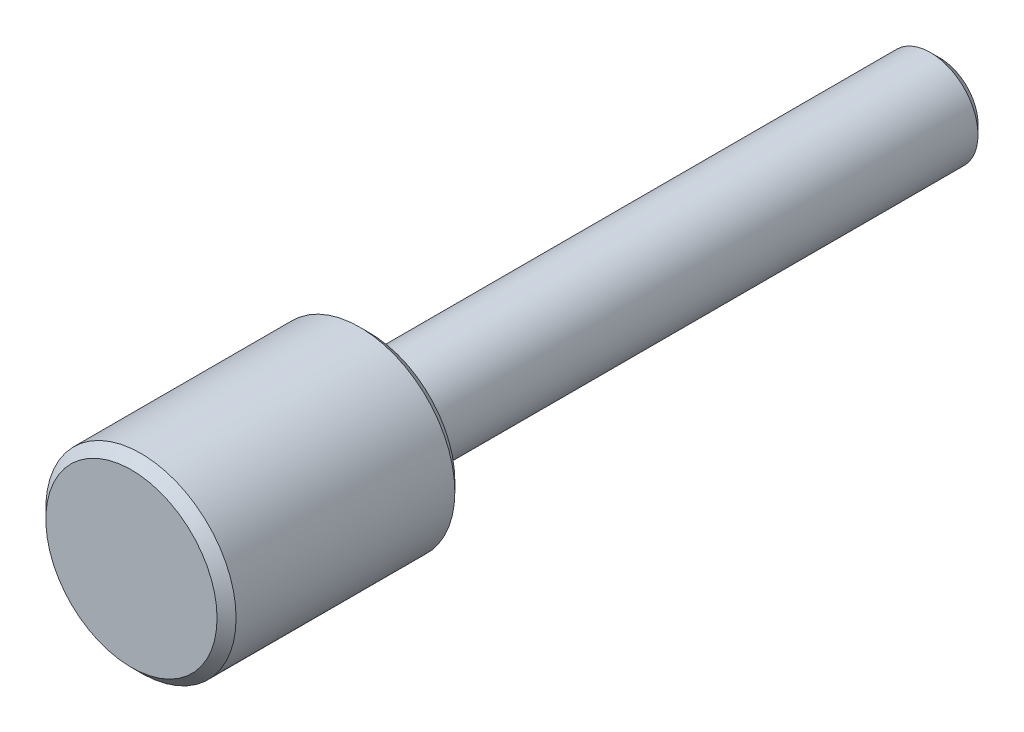
from build123d import *

# Parameters (mm, degrees)
SKETCH1_R           = 1
BOSS_EXTRUDE1_DEPTH = 8.5
SKETCH2_R           = 2
BOSS_EXTRUDE2_DEPTH = 5
CHAMFER1_SIZE       = 0.2


with BuildPart() as part:
    # Sketch1 → Boss-Extrude1 (new, symmetric)
    with BuildSketch(Plane.XY):
        Circle(SKETCH1_R)
    extrude(amount=BOSS_EXTRUDE1_DEPTH, both=True)

    # Sketch2 → Boss-Extrude2 (add)
    with BuildSketch(Plane.XY.offset(8.5)):
        Circle(SKETCH2_R)
    extrude(amount=-BOSS_EXTRUDE2_DEPTH)

    # Chamfer1
    chamfer1_edges = [part.edges().sort_by_distance(p)[0] for p in [
        (-1, 0, -8.5),
        (-2, 0, 8.5),
        (-2, 0, 3.5),
    ]]
    chamfer(chamfer1_edges, length=CHAMFER1_SIZE)


solid = part.part
